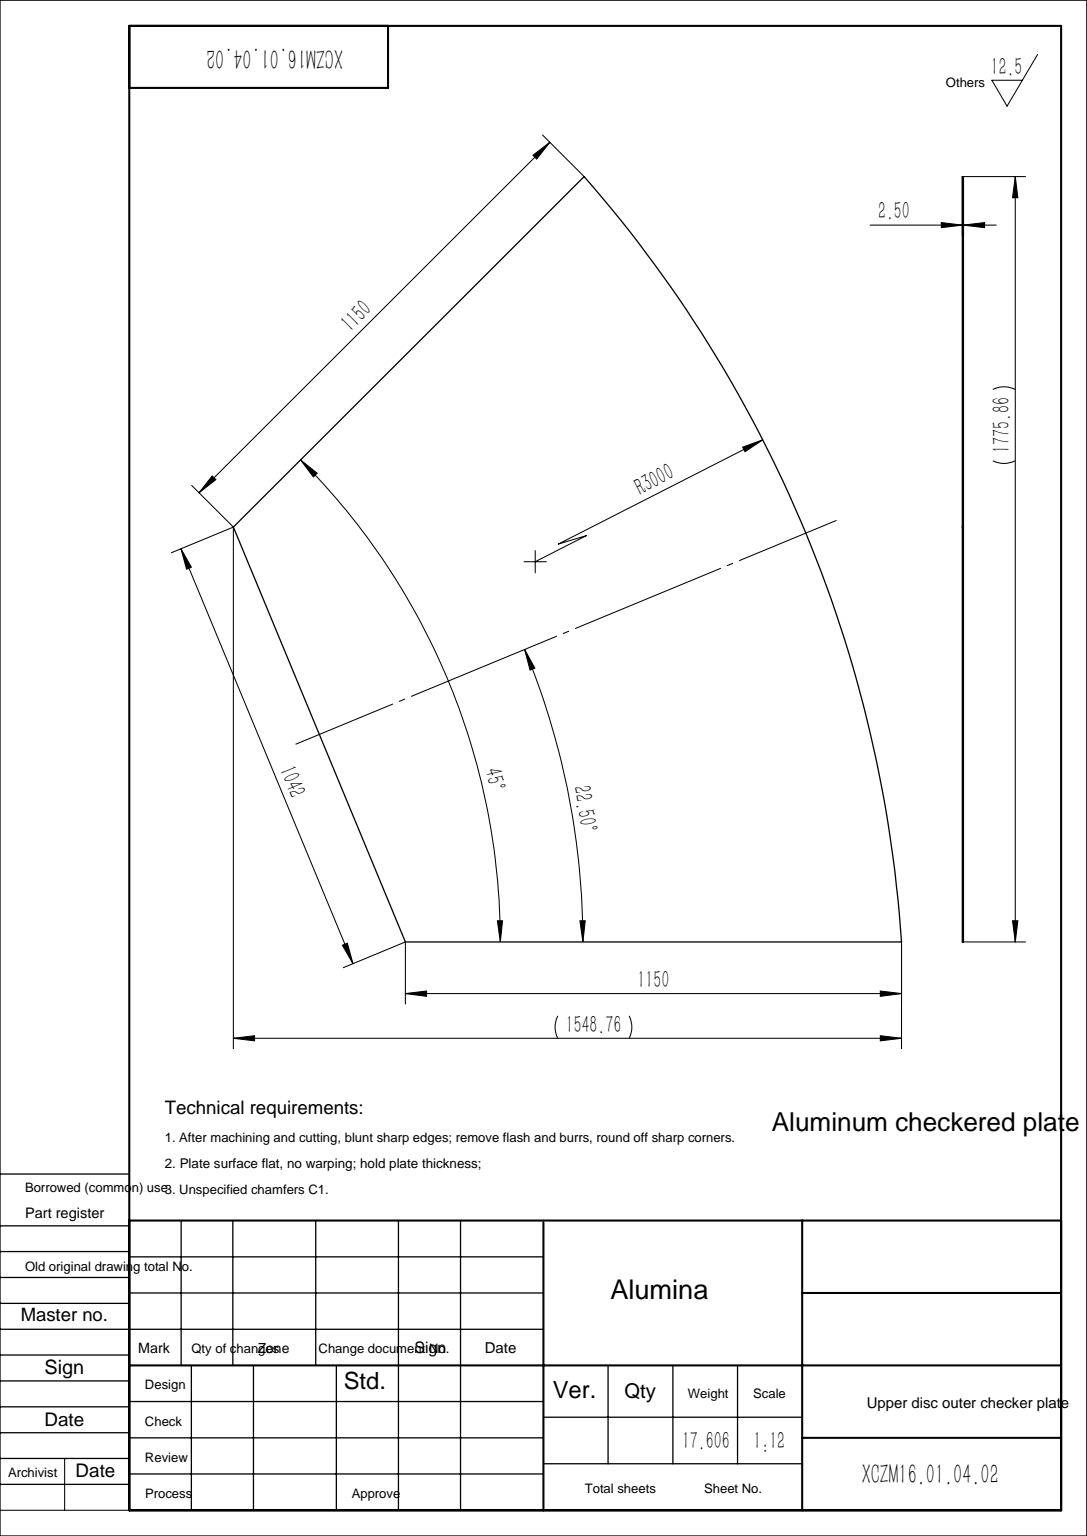
from build123d import *

# Parameters (mm, degrees)
BOSS_EXTRUDE2_DEPTH = 2.5


with BuildPart() as part:
    # Sketch2 → Boss-Extrude2 (new body)
    with BuildSketch(Plane(origin=(0, 0, 0), x_dir=(1, 0, 0), z_dir=(0, 1, 0))):
        with BuildLine():
            Line((0, 0), (-398.756136524, 962.682472877))
            Line((-398.756136524, 962.682472877), (414.41666184, 1775.855271241))
            ThreePointArc((414.41666184, 1775.855271241), (928.286982606, 948.435394322), (1150, 0))
            Line((1150, 0), (0, 0))
        make_face()
    extrude(amount=BOSS_EXTRUDE2_DEPTH)


solid = part.part
